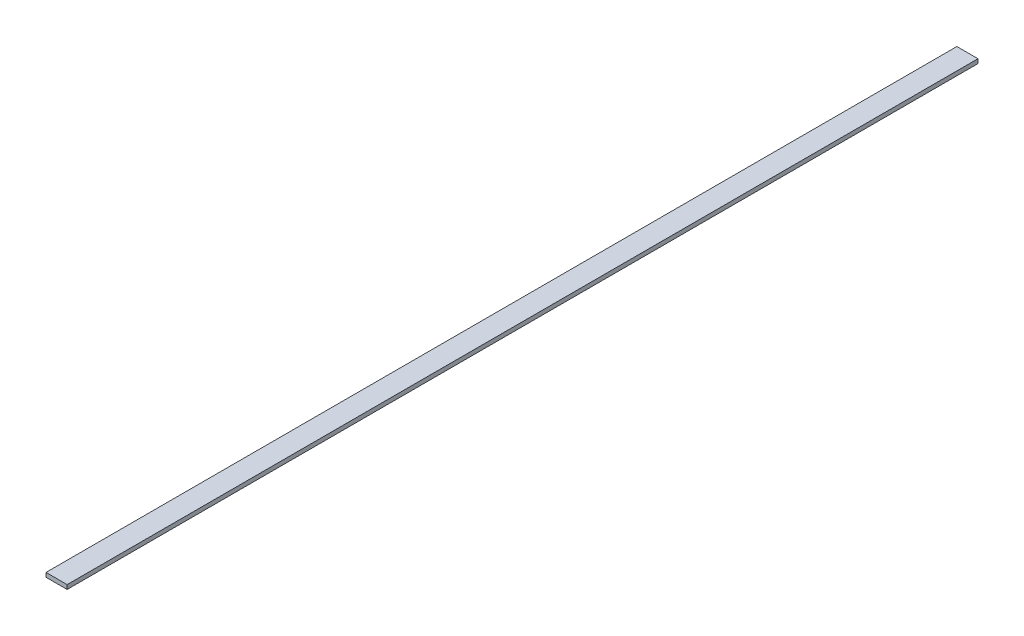
from build123d import *

# Parameters (mm, degrees)
SKETCH1_W           = 70
SKETCH1_H           = 14
BOSS_EXTRUDE1_DEPTH = 3017.15


with BuildPart() as part:
    # Sketch1 → Boss-Extrude1 (new body)
    with BuildSketch(Plane.XY):
        Rectangle(SKETCH1_W, SKETCH1_H)
    extrude(amount=BOSS_EXTRUDE1_DEPTH)


solid = part.part
